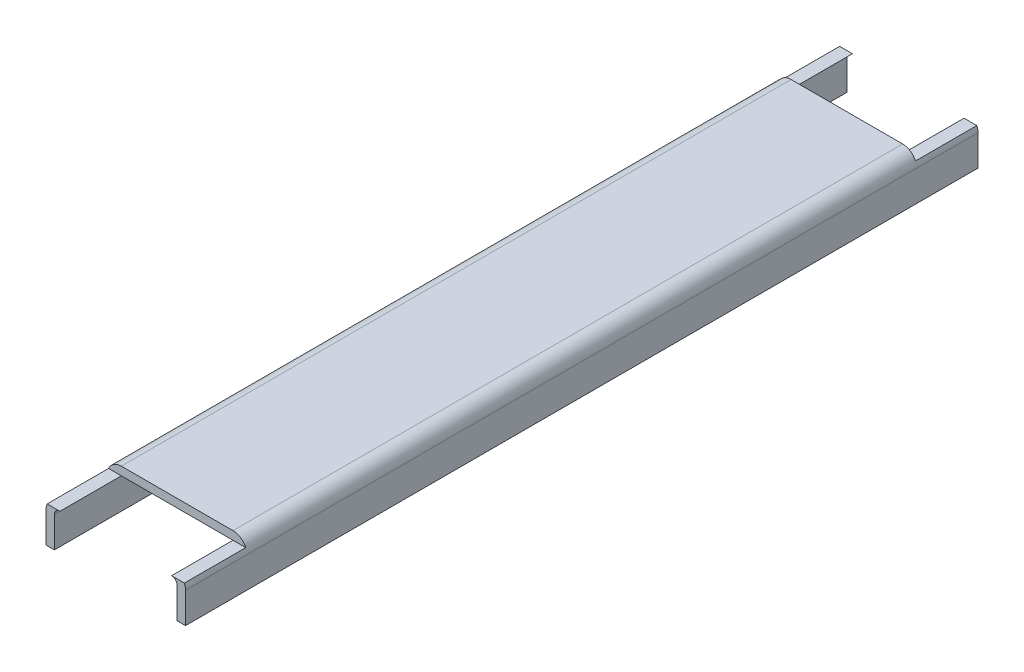
SolidWorks part; units mm, degrees
material "1023 carbon steel plate (SS)"
ref_plane "Front Plane" through (0, 0, 0) normal (0, 0, 1) x (1, 0, 0)
ref_plane "Top Plane" through (0, 0, 0) normal (0, 1, 0) x (1, 0, 0)
ref_plane "Right Plane" through (0, 0, 0) normal (1, 0, 0) x (0, 0, -1)
sketch "Sketch1" plane through (0, 0, 0) normal (0, 0, 1) x (1, 0, 0)
  line L0 (0, 0) -> (0, 22)
  line L1 (10, 32) -> (90, 32)
  line L2 (100, 22) -> (100, 0)
  line L3 (6, 0) -> (6, 22)
  line L4 (10, 26) -> (90, 26)
  line L5 (94, 22) -> (94, 0)
  line L6 (6, 0) -> (0, 0)
  line L7 (94, 0) -> (100, 0)
  arc A0 (90, 32) -> (100, 22) centre (90, 22) cw
  arc A1 (0, 22) -> (10, 32) centre (10, 22) cw
  arc A2 (6, 22) -> (10, 26) centre (10, 22) cw
  arc A3 (90, 26) -> (94, 22) centre (90, 22) cw
  point P7 (100, 32)
  point P10 (0, 32)
  dimension "D4" = 10
  dimension "D1" = 100
  dimension "D2" = 32
  dimension "D3" = 32
  dimension "D5" = 6
extrude "Boss-Extrude1" add sketch "Sketch1" along normal blind 568 contours L7 L2 A0 L1 A1 L0 L6 L3 A2 L4 A3 L5
sketch "Sketch2" plane through (0, 0, 568) normal (0, 0, 1) x (1, 0, 0)
  line L0 (-5.0167, 26) -> (110.5896, 26)
  line L1 (110.5896, 26) -> (113.5428, 46.1177)
  line L2 (113.5428, 46.1177) -> (4.0968, 46.1177)
  line L3 (4.0968, 46.1177) -> (-12.0204, 28.6158)
  line L4 (-12.0204, 28.6158) -> (-5.0167, 26)
  line L5 (10, 32) -> (90, 32) construction
  dimension "D1" = 6
extrude "Cut-Extrude1" cut sketch "Sketch2" against normal blind 44
sketch "Sketch3" plane through (0, 0, 0) normal (0, 0, -1) x (-1, 0, 0)
  line L0 (-112.0204, 26) -> (27.4665, 26)
  line L1 (27.4665, 26) -> (17.252, 45.4921)
  line L2 (17.252, 45.4921) -> (-47.8905, 56.0398)
  line L3 (-47.8905, 56.0398) -> (-51.5189, 56.0398)
  line L4 (-112.0204, 26) -> (-99.2436, 54.2054)
  line L5 (-99.2436, 54.2054) -> (-51.5189, 56.0398)
  line L7 (-10, 32) -> (-90, 32) construction
  dimension "D1" = 6
extrude "Cut-Extrude2" cut sketch "Sketch3" against normal blind 44
